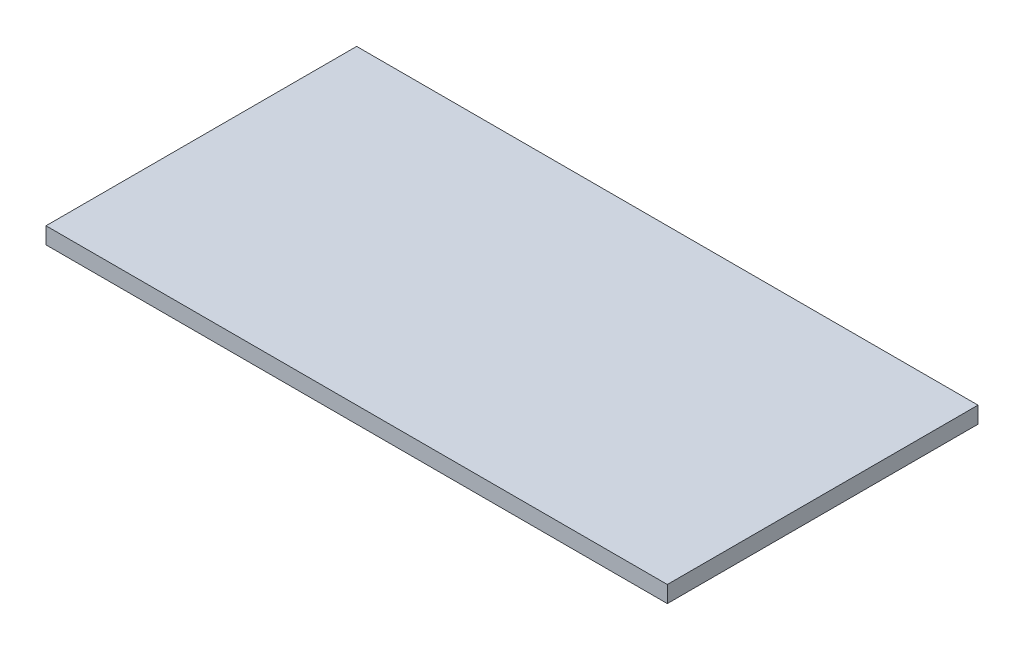
SolidWorks part; units mm, degrees
ref_plane "Front Plane" through (0, 0, 0) normal (0, 0, 1) x (1, 0, 0)
ref_plane "Top Plane" through (0, 0, 0) normal (0, 1, 0) x (1, 0, 0)
ref_plane "Right Plane" through (0, 0, 0) normal (1, 0, 0) x (0, 0, -1)
sketch "Sketch1" plane through (0, 0, 0) normal (0, 1, 0) x (1, 0, 0)
  line L1 (-300, 150) -> (300, 150)
  line L2 (-300, 150) -> (-300, -150)
  line L3 (-300, -150) -> (300, -150)
  line L4 (300, 150) -> (300, -150)
  line L5 (-300, 150) -> (300, -150) construction
  line L6 (-300, -150) -> (300, 150) construction
  point P0 (0, 0)
  dimension "D1" = 600
  dimension "D2" = 300
extrude "Boss-Extrude1" add sketch "Sketch1" along normal blind 20
sketch "Sketch2" plane through (0, 0, 0) normal (0, -1, 0) x (1, 0, 0)
  line L0 (-300, 150) -> (300, 150) construction
  line L1 (-290, 140) -> (290, 140)
  line L2 (-290, 140) -> (-290, -140)
  line L3 (-290, -140) -> (290, -140)
  line L4 (290, 140) -> (290, -140)
  line L5 (-290, 140) -> (290, -140) construction
  line L6 (-290, -140) -> (290, 140) construction
  line L7 (-300, -150) -> (-300, 150) construction
  point P0 (0, 0)
  dimension "D1" = 10
  dimension "D2" = 10
extrude "Cut-Extrude1" cut sketch "Sketch2" against normal blind 4 flip side to cut
